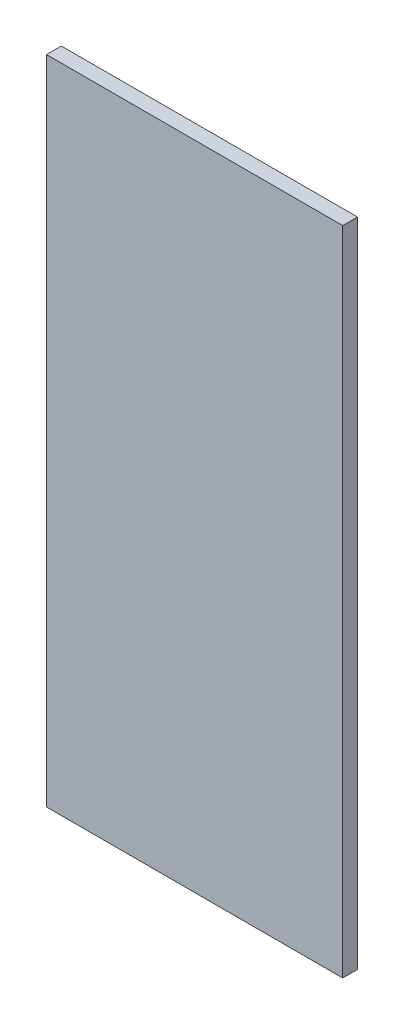
from build123d import *

# Parameters (mm, degrees)
SKETCH_1_W      = 100
SKETCH_1_H      = 220
EXTRUDE_1_DEPTH = 5


with BuildPart() as part:
    # 草图1 → 凸台-拉伸1 (new body)
    with BuildSketch(Plane.XY):
        Rectangle(SKETCH_1_W, SKETCH_1_H)
    extrude(amount=EXTRUDE_1_DEPTH)


solid = part.part
